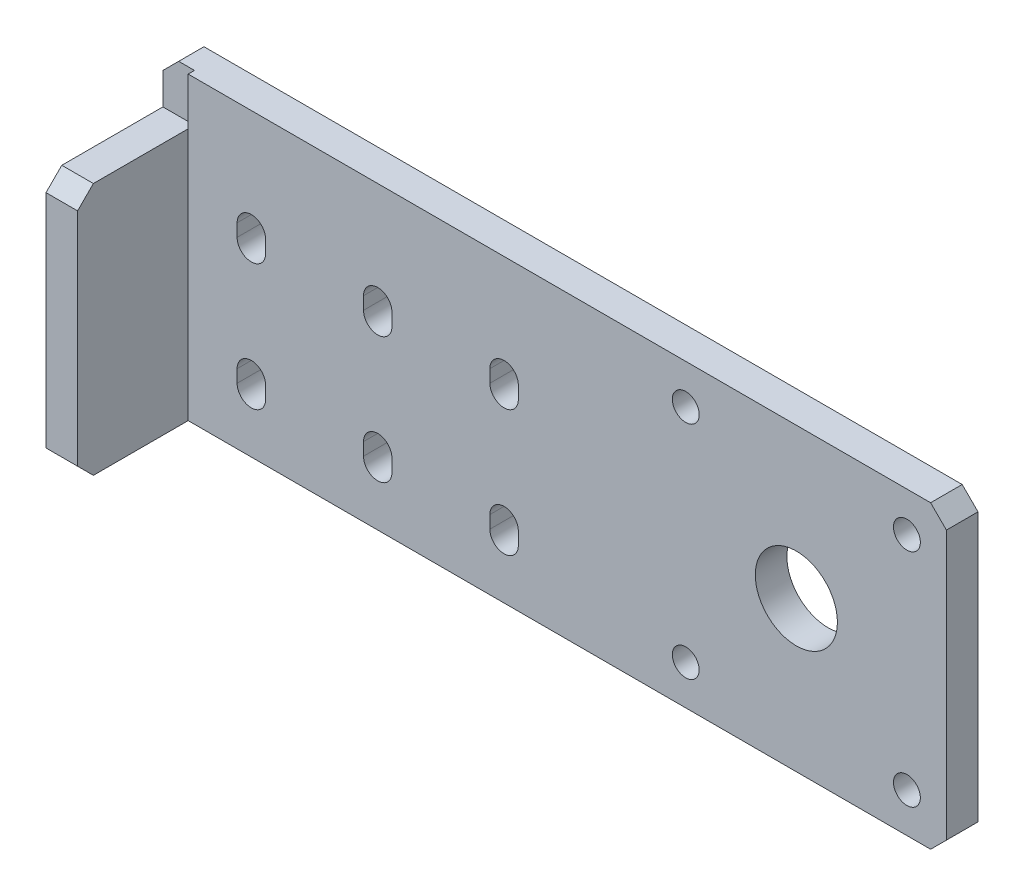
from build123d import *

# Parameters (mm, degrees)
SKETCH_1_W                  = 250
SKETCH_1_H                  = 95
EXTRUDE_1_DEPTH             = 10
CUT_EXTRUDE_2_DEPTH         = 135.094183319
PATTERN_LINEAR_1_COUNT      = 2
PATTERN_LINEAR_1_PITCH      = 40
PATTERN_LINEAR_1_COUNT_DIR2 = 2
PATTERN_LINEAR_1_PITCH_DIR2 = 40
PATTERN_LINEAR_2_COUNT      = 2
PATTERN_LINEAR_2_PITCH      = 40
PATTERN_LINEAR_2_COUNT_DIR2 = 2
PATTERN_LINEAR_2_PITCH_DIR2 = 40
HOLE_WIZARD_M10_3_D         = 8.5
HOLE_WIZARD_M10_3_DEPTH     = 24.5
HOLE_WIZARD_M10_3_TIP       = 2.553657631
SKETCH_12_R                 = 13
CUT_EXTRUDE_5_DEPTH         = 135.094183319
HOLE_WIZARD_M4_1_D          = 3.3
HOLE_WIZARD_M4_1_DEPTH      = 10.1
HOLE_WIZARD_M4_1_TIP        = 0.991420021
SKETCH_22_W                 = 10
SKETCH_22_H                 = 95
CUT_EXTRUDE_6_DEPTH         = 2
SKETCH_21_W                 = 10
SKETCH_21_H                 = 80
EXTRUDE_2_DEPTH             = 37
CHAMFER_1_SIZE              = 5
CHAMFER_2_SIZE              = 5


with BuildPart() as part:
    # 草图1 → 凸台-拉伸1 (new body)
    with BuildSketch(Plane.XY):
        Rectangle(SKETCH_1_W, SKETCH_1_H)
    extrude(amount=EXTRUDE_1_DEPTH)

    # 草图3 → 切除-拉伸2 (cut, through all)
    with BuildSketch(Plane.XY.offset(10)):
        with BuildLine():
            Line((-59.5, -29.5), (-59.5, -25.5))
            ThreePointArc((-59.5, -25.5), (-55, -21), (-50.5, -25.5))
            Line((-50.5, -25.5), (-50.5, -29.5))
            ThreePointArc((-50.5, -29.5), (-55, -34), (-59.5, -29.5))
        make_face()
    cut_extrude_2 = extrude(amount=-CUT_EXTRUDE_2_DEPTH, mode=Mode.SUBTRACT)

    # 阵列(线性)1: Cut-Extrude 2 2 × 2
    with Locations(*[(i * PATTERN_LINEAR_1_PITCH, j * PATTERN_LINEAR_1_PITCH_DIR2, 0) for i in range(PATTERN_LINEAR_1_COUNT) for j in range(PATTERN_LINEAR_1_COUNT_DIR2) if (i, j) != (0, 0)]):
        add(cut_extrude_2, mode=Mode.SUBTRACT)

    # 阵列(线性)2: Cut-Extrude 2 2 × 2
    with Locations(*[(-i * PATTERN_LINEAR_2_PITCH, j * PATTERN_LINEAR_2_PITCH_DIR2, 0) for i in range(PATTERN_LINEAR_2_COUNT) for j in range(PATTERN_LINEAR_2_COUNT_DIR2) if (i, j) != (0, 0)]):
        add(cut_extrude_2, mode=Mode.SUBTRACT)

    # M10 螺纹孔3
    with Locations(Plane(origin=(42.5, 35, 10), x_dir=(1, 0, 0), z_dir=(0, 0, 1))):
        with Locations((0, 0), (70, 0), (70, -70), (0, -70)):
            Hole(HOLE_WIZARD_M10_3_D / 2, depth=HOLE_WIZARD_M10_3_DEPTH)
            with Locations((0, 0, -(HOLE_WIZARD_M10_3_DEPTH + HOLE_WIZARD_M10_3_TIP / 2))):  # 118° drill point
                Cone(0, HOLE_WIZARD_M10_3_D / 2, HOLE_WIZARD_M10_3_TIP, mode=Mode.SUBTRACT)

    # 草图12 → 切除-拉伸5 (cut, through all)
    with BuildSketch(Plane.XY.offset(10)):
        with Locations((77.5, 0)):
            Circle(SKETCH_12_R)
    extrude(amount=-CUT_EXTRUDE_5_DEPTH, mode=Mode.SUBTRACT)

    # M4 螺纹孔1
    with Locations(Plane(origin=(117, -47.5, 5), x_dir=(0, 0, -1), z_dir=(0, -1, 0))):
        with Locations((0, 0), (0, -105), (0, -52.5)):
            Hole(HOLE_WIZARD_M4_1_D / 2, depth=HOLE_WIZARD_M4_1_DEPTH)
            with Locations((0, 0, -(HOLE_WIZARD_M4_1_DEPTH + HOLE_WIZARD_M4_1_TIP / 2))):  # 118° drill point
                Cone(0, HOLE_WIZARD_M4_1_D / 2, HOLE_WIZARD_M4_1_TIP, mode=Mode.SUBTRACT)

    # 草图22 → 切除-拉伸6 (cut)
    with BuildSketch(Plane.XY.offset(10)):
        with Locations((-120, 0)):
            Rectangle(SKETCH_22_W, SKETCH_22_H)
    extrude(amount=-CUT_EXTRUDE_6_DEPTH, mode=Mode.SUBTRACT)

    # 倒角1
    chamfer_1_edges = [part.edges().sort_by_distance(p)[0] for p in [
        (-125, 47.5, 4),
        (125, -47.5, 5),
        (125, 47.5, 5),
    ]]
    chamfer(chamfer_1_edges, length=CHAMFER_1_SIZE)


with BuildPart() as body_2:
    # 草图21 → 凸台-拉伸2 (new body)
    with BuildSketch(Plane(origin=(0, 0, 8), x_dir=(-1, 0, 0), z_dir=(0, 0, -1))):
        with Locations((120, -7.5)):
            Rectangle(SKETCH_21_W, SKETCH_21_H)
    extrude(amount=-EXTRUDE_2_DEPTH)

    # 倒角2
    chamfer_2_edges = [body_2.edges().sort_by_distance(p)[0] for p in [
        (-120, -47.5, 45),
        (-120, 32.5, 45),
    ]]
    chamfer(chamfer_2_edges, length=CHAMFER_2_SIZE)


solid = Compound([part.part, body_2.part])
